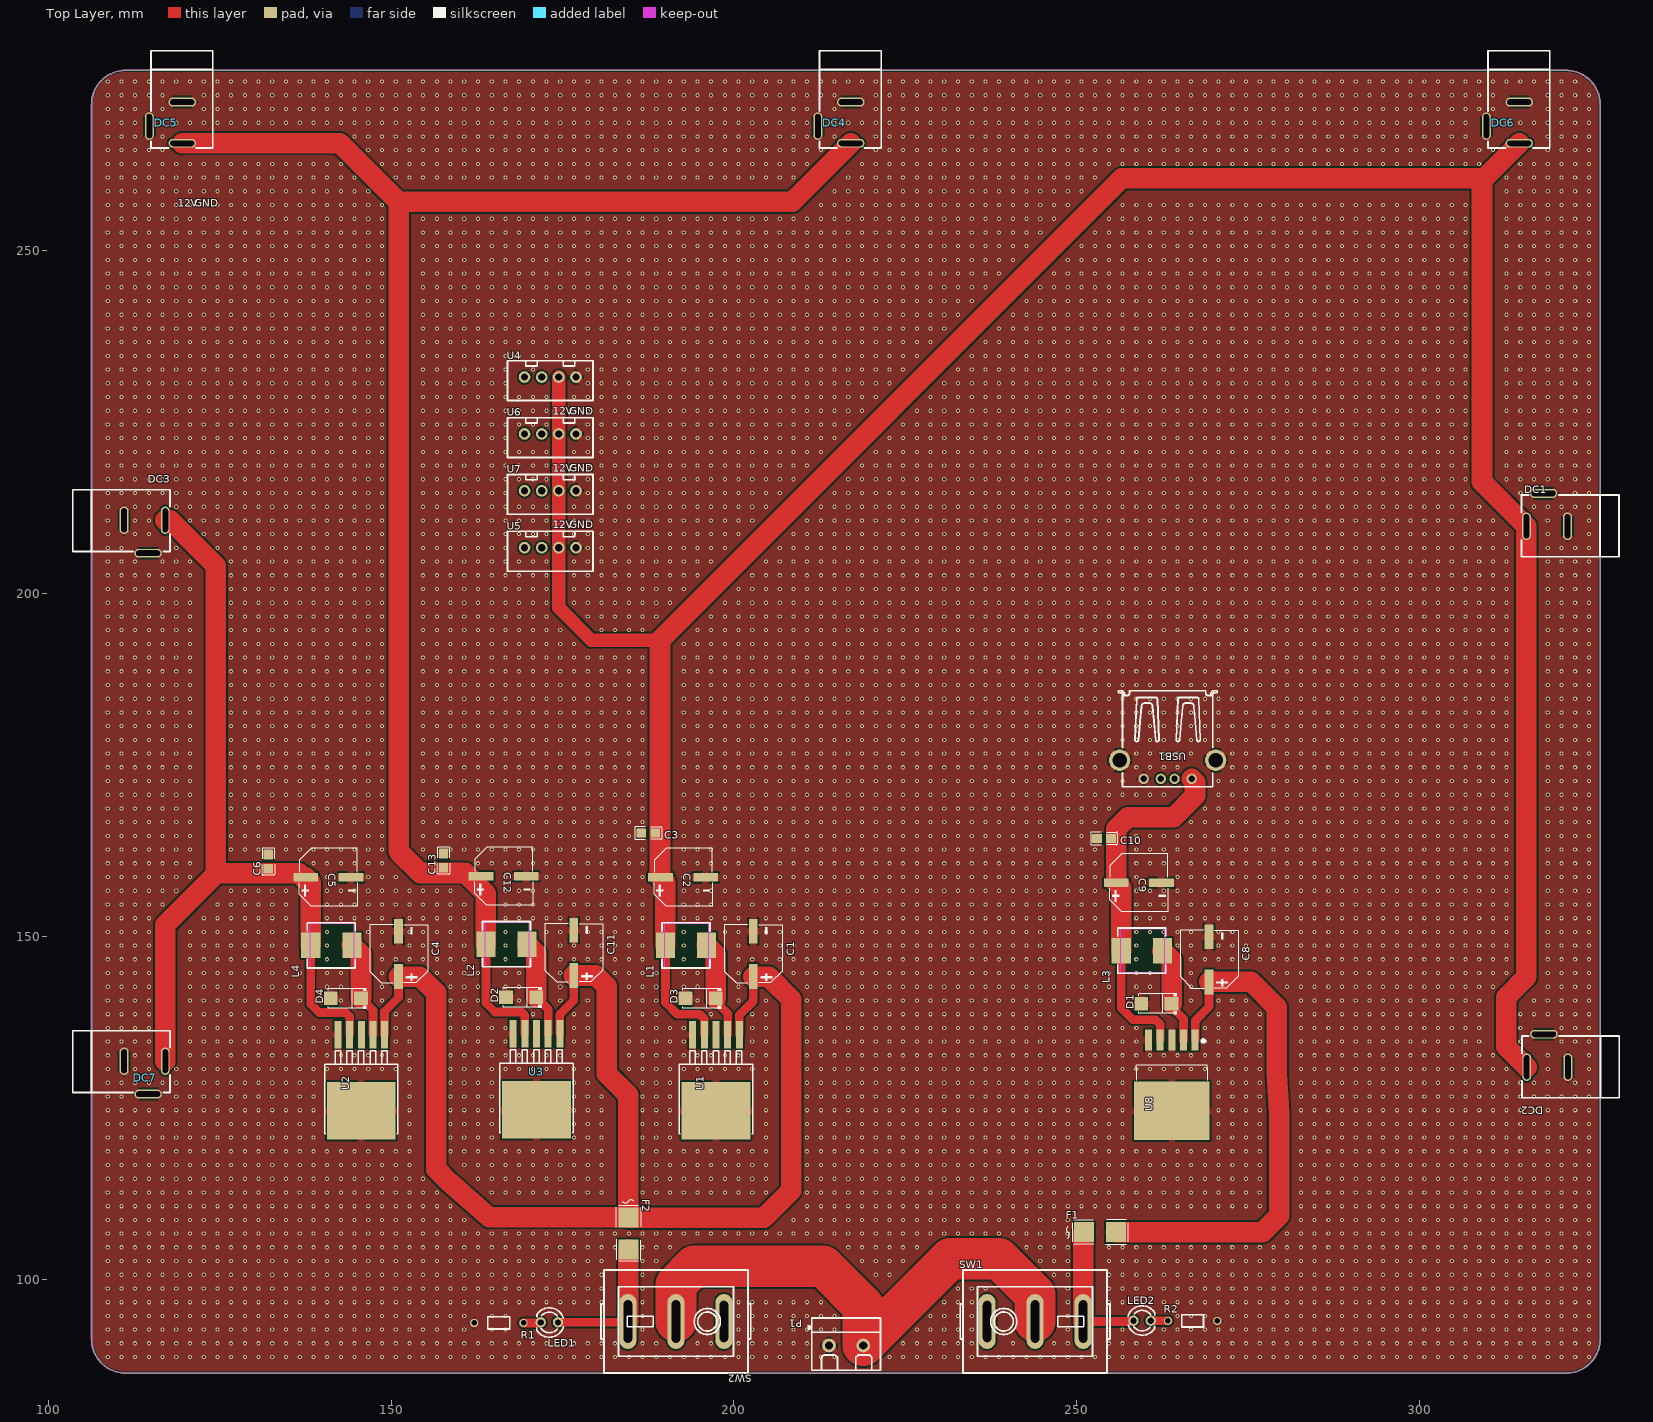
[diagram p0: Top Layer view]
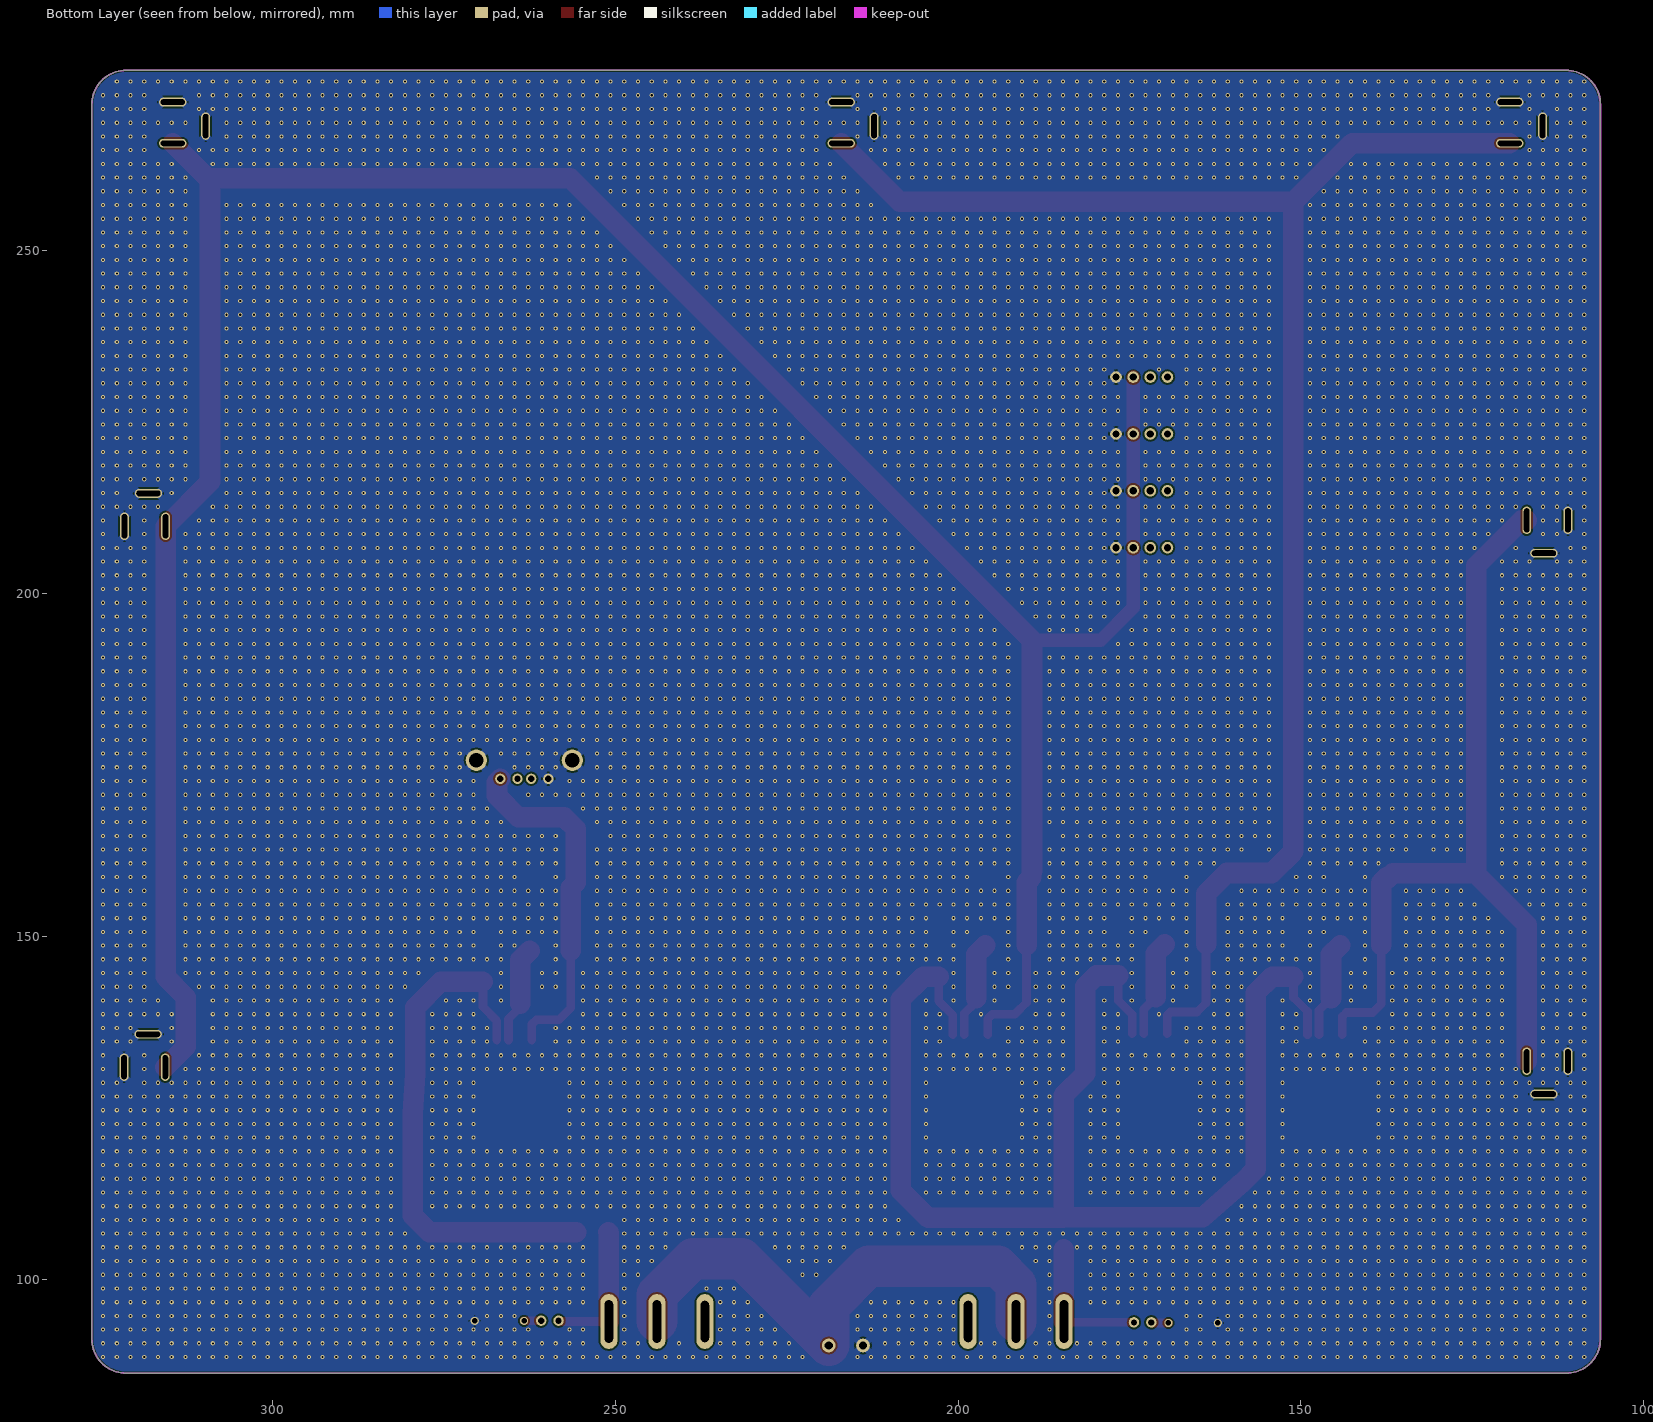
[diagram p1: Bottom Layer view, seen from below]
# Altium PCB MISC49942.pcbdoc (part 1 of 4)
Units mm, origin at the board's own origin, x right, y up, seen from the top; angles counter-clockwise.
Board outline 220 x 190 mm, 2 copper layers (Top Layer, Bottom Layer), stack 1.58 mm thick; 45 components, 14 nets, 127 pads, 8689 vias.

## Layer stack, top to bottom
Top Solder Mask Layer: solder mask 0.01, Dk 3.3
Top Layer: signal copper 0.035
Dielectric1: surface 1.51, FR4, Dk 4.5
Bottom Layer: signal copper 0.035
Bottom Solder Mask Layer: solder mask 0.01, Dk 3.3

## Board outline
111.326,276.31 ccw(c111.326,271.31) 106.326,271.31 106.326,91.31 ccw(c111.326,91.31) 111.326,86.31 321.326,86.31 ccw(c321.326,91.31) 326.326,91.31 326.326,271.31 ccw(c321.326,271.31) 321.326,276.31 111.326,276.31

## Design rules (kind name [scope] priority, off if disabled: settings)
BoardOutlineClearance copperThickness2oz_1 [All] p2 off: genericclearance=0.203 ignorepadtopadclearanceinfootprint=FALSE except(0: Arc-SplitContinuation Track-SplitContinuation SMDPad-SplitContinuation THPad-SplitContinuation Via-SplitContinuation Fill-SplitContinuation Region-SplitContinuation Poly-SplitContinuation Text-SplitContinuation Hole-SplitContinuation; 0.152: SMDPad-CutoutEdge THPad-CutoutEdge Via-CutoutEdge Fill-CutoutEdge Region-CutoutEdge Text-CutoutEdge Hole-CutoutEdge; 0.254: Poly-OutlineEdge Poly-CutoutEdge; 0.3: Arc-OutlineEdge Track-OutlineEdge SMDPad-OutlineEdge THPad-OutlineEdge Via-OutlineEdge Fill-OutlineEdge Region-OutlineEdge Text-OutlineEdge Hole-OutlineEdge Arc-CutoutEdge Track-CutoutEdge)
BoardOutlineClearance Plane_innerPlane_1 [All] p4 off: genericclearance=0.102 ignorepadtopadclearanceinfootprint=FALSE except(0: Arc-SplitContinuation Track-SplitContinuation SMDPad-SplitContinuation THPad-SplitContinuation Via-SplitContinuation Fill-SplitContinuation Region-SplitContinuation Poly-SplitContinuation Text-SplitContinuation Hole-SplitContinuation; 0.152: SMDPad-CutoutEdge THPad-CutoutEdge Via-CutoutEdge Fill-CutoutEdge Region-CutoutEdge Text-CutoutEdge Hole-CutoutEdge; 0.254: Poly-OutlineEdge Poly-CutoutEdge; 0.3: Arc-OutlineEdge Track-OutlineEdge SMDPad-OutlineEdge THPad-OutlineEdge Via-OutlineEdge Fill-OutlineEdge Region-OutlineEdge Text-OutlineEdge Hole-OutlineEdge Arc-CutoutEdge Track-CutoutEdge)
BoardOutlineClearance Copper_copperRegion_1 [All] p6 off: genericclearance=0.102 ignorepadtopadclearanceinfootprint=FALSE except(0: Arc-SplitContinuation Track-SplitContinuation SMDPad-SplitContinuation THPad-SplitContinuation Via-SplitContinuation Fill-SplitContinuation Region-SplitContinuation Poly-SplitContinuation Text-SplitContinuation Hole-SplitContinuation; 0.152: SMDPad-CutoutEdge THPad-CutoutEdge Via-CutoutEdge Fill-CutoutEdge Region-CutoutEdge Text-CutoutEdge Hole-CutoutEdge; 0.254: Poly-OutlineEdge Poly-CutoutEdge; 0.3: Arc-OutlineEdge Track-OutlineEdge SMDPad-OutlineEdge THPad-OutlineEdge Via-OutlineEdge Fill-OutlineEdge Region-OutlineEdge Text-OutlineEdge Hole-OutlineEdge Arc-CutoutEdge Track-CutoutEdge)
BoardOutlineClearance copperThickness1oz_1 [All] p8: genericclearance=0.102 ignorepadtopadclearanceinfootprint=FALSE except(0: Arc-SplitContinuation Track-SplitContinuation SMDPad-SplitContinuation THPad-SplitContinuation Via-SplitContinuation Fill-SplitContinuation Region-SplitContinuation Poly-SplitContinuation Text-SplitContinuation Hole-SplitContinuation; 0.152: SMDPad-CutoutEdge THPad-CutoutEdge Via-CutoutEdge Fill-CutoutEdge Region-CutoutEdge Text-CutoutEdge Hole-CutoutEdge; 0.254: Poly-OutlineEdge Poly-CutoutEdge; 0.3: Arc-OutlineEdge Track-OutlineEdge SMDPad-OutlineEdge THPad-OutlineEdge Via-OutlineEdge Fill-OutlineEdge Region-OutlineEdge Text-OutlineEdge Hole-OutlineEdge Arc-CutoutEdge Track-CutoutEdge)
Clearance copperThickness2oz [All] p1 off: gap=0.203 ignorepadtopadclearanceinfootprint=FALSE except(0.152: SMDPad-Track SMDPad-SMDPad THPad-Track SMDPad-THPad THPad-THPad Track-Via SMDPad-Via THPad-Via Via-Via Fill-Track Region-Track Fill-SMDPad Region-SMDPad Fill-THPad Region-THPad Fill-Via Region-Via Fill-Fill Fill-Region Region-Region Arc-Track Arc-SMDPad Arc-THPad Arc-Via Fill-Arc Region-Arc Arc-Arc Text-Track SMDPad-Text Text-THPad Text-Via Fill-Text Region-Text Arc-Text Text-Text Hole-Track Hole-SMDPad Hole-THPad Hole-Via Fill-Hole Region-Hole Hole-Arc Hole-Text; 0.254: Poly-Track Poly-SMDPad Poly-THPad Poly-Via Poly-Fill Poly-Region Poly-Poly Poly-Arc Poly-Text Poly-Hole)
Clearance Plane_innerPlane [All] p3 off: gap=0.102 ignorepadtopadclearanceinfootprint=FALSE except(0.152: SMDPad-Track SMDPad-SMDPad THPad-Track SMDPad-THPad THPad-THPad Track-Via SMDPad-Via THPad-Via Via-Via Fill-Track Region-Track Fill-SMDPad Region-SMDPad Fill-THPad Region-THPad Fill-Via Region-Via Fill-Fill Fill-Region Region-Region Arc-Track Arc-SMDPad Arc-THPad Arc-Via Fill-Arc Region-Arc Arc-Arc Text-Track SMDPad-Text Text-THPad Text-Via Fill-Text Region-Text Arc-Text Text-Text Hole-Track Hole-SMDPad Hole-THPad Hole-Via Fill-Hole Region-Hole Hole-Arc Hole-Text; 0.254: Poly-Track Poly-SMDPad Poly-THPad Poly-Via Poly-Fill Poly-Region Poly-Poly Poly-Arc Poly-Text Poly-Hole)
Clearance Copper_copperRegion [All] p5 off: gap=0.102 ignorepadtopadclearanceinfootprint=FALSE except(0.152: SMDPad-Track SMDPad-SMDPad THPad-Track SMDPad-THPad THPad-THPad Track-Via SMDPad-Via THPad-Via Via-Via Fill-Track Region-Track Fill-SMDPad Region-SMDPad Fill-THPad Region-THPad Fill-Via Region-Via Fill-Fill Fill-Region Region-Region Arc-Track Arc-SMDPad Arc-THPad Arc-Via Fill-Arc Region-Arc Arc-Arc Text-Track SMDPad-Text Text-THPad Text-Via Fill-Text Region-Text Arc-Text Text-Text Hole-Track Hole-SMDPad Hole-THPad Hole-Via Fill-Hole Region-Hole Hole-Arc Hole-Text; 0.254: Poly-Track Poly-SMDPad Poly-THPad Poly-Via Poly-Fill Poly-Region Poly-Poly Poly-Arc Poly-Text Poly-Hole)
Clearance copperThickness1oz [All] p7: gap=0.102 ignorepadtopadclearanceinfootprint=FALSE except(0.152: SMDPad-Track SMDPad-SMDPad THPad-Track SMDPad-THPad THPad-THPad Track-Via SMDPad-Via THPad-Via Via-Via Fill-Track Region-Track Fill-SMDPad Region-SMDPad Fill-THPad Region-THPad Fill-Via Region-Via Fill-Fill Fill-Region Region-Region Arc-Track Arc-SMDPad Arc-THPad Arc-Via Fill-Arc Region-Arc Arc-Arc Text-Track SMDPad-Text Text-THPad Text-Via Fill-Text Region-Text Arc-Text Text-Text Hole-Track Hole-SMDPad Hole-THPad Hole-Via Fill-Hole Region-Hole Hole-Arc Hole-Text; 0.254: Poly-Track Poly-SMDPad Poly-THPad Poly-Via Poly-Fill Poly-Region Poly-Poly Poly-Arc Poly-Text Poly-Hole)
DiffPairsRouting differentialPair [All] p1: maxlimit=0.152 minlimit=0.152 mostfreqgap=0.152 toplayer_minwidth=0.127 toplayer_prefwidth=0.254 toplayer_maxwidth=2.54 toplayer_mingap=0.152 toplayer_prefgap=0.152 toplayer_maxgap=0.152 bottomlayer_minwidth=0.127 bottomlayer_prefwidth=0.254 bottomlayer_maxwidth=2.54 bottomlayer_mingap=0.152 bottomlayer_prefgap=0.152 bottomlayer_maxgap=0.152 maxuncoupledlength=0.254
HoleToHoleClearance otherClearance [All] p1: gap=0.3 allowstackedmicrovias=TRUE
Length netLength [All] p1: minlimit=0 maxlimit=0
MatchedLengths netLengthTolerance [All] p1: tolerance=25.4
PasteMaskExpansion pasteMaskExpansion [All] p1: expansion=0
PlaneConnect innerPlane [All] p1: planeconnectstyle=Relief reliefexpansion=0.508 reliefentries=4 reliefconductorwidth=0.254 reliefairgap=0.254
PolygonConnect copperRegion [All] p1: connectstyle=Relief reliefconductorwidth=1 reliefentries=4 polygonreliefangle="45 Angle" airgapwidth=0.254 smdpad.connectstyle=Relief smdpad.reliefconductorwidth=1 smdpad.reliefentries=4 smdpad.polygonreliefangle="90 Angle" smdpad.airgapwidth=0.254 via.connectstyle=Relief via.reliefconductorwidth=0.254 via.reliefentries=4 via.polygonreliefangle="90 Angle" via.airgapwidth=0.254
RoutingVias viaSize [All] p1: holewidth=0.305 width=0.61 viastyle="Through Hole" minholewidth=0.3 minwidth=0.5 maxholewidth=6.3 maxwidth=10
SolderMaskExpansion solderMaskExpansion [IsVia] p1: expansion=-25.4 istentingtop=TRUE
SolderMaskExpansion solderMaskExpansion [All] p2: expansion=0.051 istentingtop=FALSE
Width copperThickness2oz_2 [All] p1 off: maxlimit=2.54 minlimit=0.203 preferedwidth=0.254
Width copperThickness1oz_2 [All] p2: maxlimit=0.254 minlimit=0.254 preferedwidth=0.254 toplayer_minwidth=0.127 toplayer_maxwidth=5.999 toplayer_prefwidth=0.254 bottomlayer_minwidth=0.127 bottomlayer_maxwidth=5.999 bottomlayer_prefwidth=0.254

## Components (designator, comment, footprint, x,y, rotation, side; value= is the part's Value field where it differs from the comment)
C1 "" CAP-SMD_BD8.0-L8.3-W8.3-RD 202.823,147.447 r270 top
C2 "" CAP-SMD_BD8.0-L8.3-W8.3-RD 192.6,158.609 r180 top
C3 "" C0805 187.5,165.075 r180 top
C4 "" CAP-SMD_BD8.0-L8.3-W8.3-RD 151.098,147.447 r270 top
C5 "" CAP-SMD_BD8.0-L8.3-W8.3-RD 140.874,158.609 r180 top
C6 "" C0805 132.111,160.914 r90 top
C8 "" CAP-SMD_BD8.0-L8.3-W8.3-RD 269.296,146.668 r270 top
C9 "" CAP-SMD_BD8.0-L8.3-W8.3-RD 259.073,157.831 r180 top
C10 "" C0805 253.973,164.296 r180 top
C11 "" CAP-SMD_BD8.0-L8.3-W8.3-RD 176.648,147.597 r270 top
C12 "" CAP-SMD_BD8.0-L8.3-W8.3-RD 166.424,158.759 r180 top
C13 "" C0805 157.661,161.064 r90 top
D1 "" SMA_L4.3-W2.6-LS5.2-RD 261.626,140.191 r180 top
D2 "" SMA_L4.3-W2.6-LS5.2-RD 168.977,141.12 r180 top
D3 "" SMA_L4.3-W2.6-LS5.2-RD 195.153,140.97 r180 top
D4 "" SMA_L4.3-W2.6-LS5.2-RD 143.427,140.97 r180 top
DC1 "" DC-2.0 318.7,209.55 r0 top
DC2 "" DC-2.0 318.75,130.67 r0 top
DC3 "" DC-2.0 113.95,210.955 r180 top
DC4 "" DC-2.0 217.312,268.8 r90 top
DC5 "" DC-2.0 119.825,268.8 r90 top
DC6 "" DC-2.0 314.8,268.8 r90 top
DC7 "" DC-2.0 113.95,132.075 r180 top
F1 "10A保险丝" FUSE-SMD_L6.1-W2.6 253.375,106.875 r0 top
F2 "10A保险丝" FUSE-SMD_L6.1-W2.6 184.625,106.7 r270 top
L1 "" IND-SMD_L7.0-W6.6 193.019,148.717 r180 top
L2 "" IND-SMD_L7.0-W6.6 166.844,148.867 r180 top
L3 "" IND-SMD_L7.0-W6.6 259.492,147.938 r180 top
L4 "" IND-SMD_L7.0-W6.6 141.294,148.717 r180 top
LED1 "" LED_TH-3mm 173.085,93.72 r180 top
LED2 "" LED_TH-3mm 259.539,93.978 r0 top
P1 "KF301-2P接线端子" CONN-TH_XY301V-A-5.0-2P 216.372,90.35 r180 top
R1 "1kΩ" Res_1/8W 165.725,93.7 r180 top
R2 "1kΩ" Res_1/8W 266.9,93.875 r0 top
SW1 "船型开关601-10211BB" SW-TH_601-10211BB 243.925,93.85 r0 top
SW2 "船型开关601-10211BB" SW-TH_601-10211BB 191.55,93.85 r180 top
U1 "LM2596S-12" TO-263-5_L10.0-W8.4-P1.70-LS15.3-BR 197.388,130.112 r90 top
U2 "LM2596S-12" TO-263-5_L10.0-W8.4-P1.70-LS15.3-BR 145.663,130.112 r90 top
U3 "LM2596S-12" TO-263-5_L10.0-W8.4-P1.70-LS15.3-BR 171.213,130.262 r90 top
U4 "XH2.54_4P_直插" CONN-TH_4P-P2.50-XH2.54-4P 173.222,231.575 r0 top
U5 "XH2.54_4P_直插" CONN-TH_4P-P2.50-XH2.54-4P 173.222,206.7 r0 top
U6 "XH2.54_4P_直插" CONN-TH_4P-P2.50-XH2.54-4P 173.222,223.283 r0 top
U7 "XH2.54_4P_直插" CONN-TH_4P-P2.50-XH2.54-4P 173.222,214.992 r0 top
U8 "LM2596S-5.0" TO-263-5_L10.2-W8.9-P1.70-BR 263.861,129.723 r90 top
USB1 "" "USB_ Type-A" 263.275,178.45 r180 top

## Footprints (in the part's own frame and the unit in brackets; to place one, negate y for a bottom-side part, rotate by r counter-clockwise, add the part's x,y. Pads: shape width x height; smd on the part's side, far side on the other; paste and mask are expansions set on the pad)
C0805 [mm]
  rect 1.41x1.35 smd paste-100 mask+0.051: 1(-1.03,0) 2(1.03,0)
  silkscreen extent -1.96,-0.9 1.96,0.9
CAP-SMD_BD8.0-L8.3-W8.3-RD [mm]
  rect 3.61x1.26 smd paste+0 mask+0.051: 1(3.295,0) 2(-3.295,0)
  silkscreen extent -4.23,-4.23 4.23,4.23
CONN-TH_4P-P2.50-XH2.54-4P [mm]
  round 1.7 hole 1.05 paste+0 mask+0.05: 1(3.75,0) 2(1.25,0) 3(-1.25,0) 4(-3.75,0)
  silkscreen extent -6.25,-3.42 6.25,2.37
CONN-TH_XY301V-A-5.0-2P [mm]
  round 2 hole 1.2: 1(-2.5,0) 2(2.5,0)
  silkscreen extent -5,-4 5.6,3.6
DC-2.0 [mil]
  oval 157.5x51.2 hole 31.5 slot 137.8 at 0 deg paste+0 mask+2: 2(-24.7,199.5)
  oval 51.2x157.5 hole 31.5 slot 137.8 at 90 deg paste+0 mask+2: 3(113.1,10.5) 4(-123.1,10.5)
  silkscreen extent -151,-165 408,190
FUSE-SMD_L6.1-W2.6 [mm]
  rect 2.91x2.911 smd paste-100 mask+0.051: 1(-2.33,0) 2(2.33,0)
  silkscreen extent -4.89,-1.78 4.06,1.78
IND-SMD_L7.0-W6.6 [mm]
  rect 2.799x3.701 smd paste+0 mask+0.051: 1(-3,0) 2(3,0)
  silkscreen extent -3.5,-3.3 3.5,3.3
LED_TH-3mm [mil]
  round 60 hole 36 paste+0 mask+2: 1(-50,0) 2(50,0)
  silkscreen extent -81,-84 72,85
Res_1/8W [mil]
  round 47.2 hole 31.5 paste+0 mask+2: 1(-141.7,2.48) 2(141.7,2.48)
  silkscreen extent -63,-33 63,38
SMA_L4.3-W2.6-LS5.2-RD [mm]
  rect 2x2 smd paste+0 mask+0.051: 1(-2.2,0) 2(2.2,0)
  silkscreen extent -2.98,-1.5 2.6,1.5
SW-TH_601-10211BB [mm]
  oval 2.5x8 hole 1.2 slot 6 at 90 deg: 1(-7,0)
  oval 2.5x8 hole 1.2 slot 6.2 at 90 deg: 2(0,0) 3(7,0)
  silkscreen extent -10.92,-7.5 10.92,7.5
TO-263-5_L10.0-W8.4-P1.70-LS15.3-BR [mm]
  rect 4x1.02 smd: 1(5.55,-3.4) 2(5.55,-1.7) 3(5.55,0) 4(5.55,1.7) 5(5.55,3.4)
  rect 8.4x10 smd: 6(-5.55,0)
  silkscreen extent -8.91,-5.33 3.2,5.33
TO-263-5_L10.2-W8.9-P1.70-BR [mm]
  rect 3.083x1.02 smd: 1(5.16,-3.4) 2(5.16,-1.7) 3(5.16,0) 4(5.16,1.7) 5(5.16,3.4)
  rect 8.5x11 smd: 6(-5.16,0)
  silkscreen extent -0.66,-5.16 5.26,5.16
"USB_ Type-A" [mm]
  round 1.5 hole 0.9 copper offset 0,0 paste+0 mask+0.051: 1(-3.484,5.461) 4(3.516,5.461)
  round 1.5 hole 0.9 paste+0 mask+0.051: 2(-0.984,5.461) 3(1.016,5.461)
  round 3.1 hole 2.1 paste+0 mask+0.051: SH1(7.016,2.751) SH2(-6.984,2.751)
  silkscreen extent -7.2,-7.4 7.24,6.6

## Via types
v1: diameter 0.61, hole 0.305, Top Layer to Bottom Layer, 8689 vias

## Nets (pads, with @x,y where several pads share a name; then routed paths per layer and width w, separated by ;. In a path a pad name is that pad's centre, name@x,y a point inside that pad or via, vN(x,y) a via of type N, cw(c..) or ccw(c..) an arc to the next point about the centre after c; other vN are vias at no path point)
5V: C9.1 C10.1 L3.2 U8.4 USB1.1 | length 51.5
  Top Layer w1.27: L3.2@256.492,147.938 256.492,139.577 258.198,137.871 261.498,137.871 262.161,137.209 U8.4@262.161,134.883
  Top Layer w3: L3.2@256.492,147.938 256.492,157.116 C9.1@255.778,157.831 255.778,165.703 257.475,167.4 264.15,167.4 267.25,170.5 267.25,172.498 USB1.1@266.759,172.989
12V: C2.1 C3.1 C5.1 C6.1 C12.1 C13.1 DC1.4 DC2.4 DC3.4 DC4.4 DC5.4 DC6.4 DC7.4 L1.2 L2.2 L4.2 U1.4 U2.4 U3.4 U4.2 U5.2 U6.2 U7.2 | length 767.7
  Top Layer w1.27: L4.2@138.294,148.717 138.294,140.156 139.525,138.925 143.375,138.925 143.963,138.337 U2.4@143.963,135.662 ; L2.2@163.844,148.867 163.844,140.297 165.166,138.975 169.05,138.975 169.513,138.512 U3.4@169.513,135.812 ; L1.2@190.019,148.717 190.019,140.356 191.725,138.65 195.025,138.65 195.688,137.987 U1.4@195.688,135.662
  Top Layer w2: U4.2@174.472,231.575 U6.2@174.472,223.283 U7.2@174.472,214.992 U5.2@174.472,206.7 174.472,197.928 179.2,193.2 189.225,193.2
  Top Layer w3: DC7.4@117.077,131.808 117.077,151.702 124.575,159.2 136.625,159.2 137.373,158.452 138.157,158.032 C5.1@137.579,158.609 ; DC3.4@117.077,210.688 117.812,210.688 124.45,204.05 124.45,159.5 ; DC5.4@119.558,265.673 142.552,265.673 151.1,257.125 ; L4.2@138.294,148.717 138.294,157.85 ; L2.2@163.844,148.867 163.844,156.248 160.842,159.25 154.25,159.25 151.1,162.4 151.1,257.125 ; 189.225,159.55 189.225,193.2 256.575,260.55 309.41,260.55 DC6.4@314.533,265.673 ; C2.1@189.305,158.609 190.019,157.895 L1.2@190.019,148.717 ; DC4.4@217.046,265.673 208.498,257.125 151.1,257.125 ; 309.1,260.2 309.1,216.29 DC1.4@315.573,209.817 315.573,144.098 312.625,141.15 312.625,133.935 DC2.4@315.623,130.937
$1N2721: D1.1 L3.1 U8.2 | length 13.9
  Top Layer w1.27: D1.1@263.825,139.719 265.561,137.984 U8.2@265.561,134.883
  Top Layer w3: L3.1@262.492,147.938 263.825,146.605 D1.1@263.825,140.191
$1N2726: D2.1 L2.1 U3.2 | length 14.3
  Top Layer w1.27: D2.1@171.177,141.12 172.913,139.385 U3.2@172.913,135.812
  Top Layer w3: L2.1@169.844,148.867 171.177,147.533 D2.1@171.177,141.12
$1N4538: P1.1 SW1.2 SW2.2 | length 78.3
  Top Layer w6: SW2.2@191.55,93.85 191.55,99.25 194.2,101.9 213.05,101.9 218.872,96.078 P1.1@218.872,90.35 231.522,103 238.675,103 243.925,97.75 SW1.2@243.925,93.85
$1N4689: D3.1 L1.1 U1.2 | length 13.9
  Top Layer w1.27: D3.1@197.352,140.498 199.088,138.762 U1.2@199.088,135.662
  Top Layer w3: L1.1@196.019,148.717 197.352,147.383 D3.1@197.352,140.97
$1N4693: D4.1 L4.1 U2.2 | length 14.3
  Top Layer w1.27: D4.1@145.627,140.97 147.363,139.235 U2.2@147.363,135.662
  Top Layer w3: L4.1@144.294,148.717 145.627,147.383 D4.1@145.627,140.97
$1N4714: LED1.2 R1.1 | length 2.5
  Top Layer w1.27: R1.1@169.324,93.637 171.733,93.637 LED1.2@171.815,93.72
$1N4717: LED2.2 R2.1 | length 2.5
  Top Layer w1.27: LED2.2@260.809,93.978 263.261,93.978 R2.1@263.301,93.938
$1N4718: F1.1 LED2.1 SW1.3 | length 20.5
  Top Layer w1.27: SW1.3@250.925,93.85 258.141,93.85 LED2.1@258.269,93.978
  Top Layer w3: SW1.3@250.925,93.85 250.925,106.755 F1.1@251.045,106.875
$1N4719: C8.1 F1.2 U8.1 | length 75.9
  Top Layer w1.27: U8.1@267.261,134.883 267.261,137.711 269.296,139.746 C8.1@269.296,143.373
  Top Layer w3: F1.2@255.705,106.875 277.1,106.875 279.5,109.275 279.5,124.25 279.175,129.925 279.175,139.65 275.452,143.373 C8.1@269.296,143.373
$1N4720: F2.2 LED1.1 SW2.3 | length 20.6
  Top Layer w1.27: LED1.1@174.355,93.72 SW2.3@184.419,93.72
  Top Layer w3: SW2.3@184.55,93.85 184.625,93.925 F2.2@184.625,104.37
$1N4721: C1.1 C4.1 C11.1 F2.1 U1.1 U2.1 U3.1 | length 191.6
  Top Layer w1.27: U2.1@149.063,135.662 149.063,139.063 151.098,141.098 C4.1@151.098,144.152 ; U3.1@174.613,135.812 174.613,138.613 176.648,140.648 C11.1@176.648,144.302 ; U1.1@200.788,135.662 200.788,138.538 202.823,140.573 C1.1@202.823,144.152
  Top Layer w3: C4.1@151.098,144.152 154.198,144.152 156.575,141.775 156.575,116.075 158.512,114.138 164.345,109.03 F2.1@184.625,109.03 ; C11.1@176.648,144.302 179.873,144.302 181.475,142.7 181.475,129.984 184.625,126.834 F2.1@184.625,109.03 ; C1.1@202.823,144.152 205.048,144.152 208.35,140.85 208.35,112.95 204.35,108.95 184.705,108.95 F2.1@184.625,109.03
GND: C1.2 C2.2 C3.2 C4.2 C5.2 C6.2 C8.2 C9.2 C10.2 C11.2 C12.2 C13.2 D1.2 D2.2 D3.2 D4.2 DC1.2 DC1.3 DC2.2 DC2.3 DC3.2 DC3.3 DC4.2 DC4.3 DC5.2 DC5.3 DC6.2 DC6.3 DC7.2 DC7.3 P1.2 R1.2 R2.2 U1.5 U1.6 U2.5 U2.6 U3.5 U3.6 U4.1 U5.1 U6.1 U7.1 U8.3 U8.5 U8.6 USB1.4 USB1.SH1 USB1.SH2